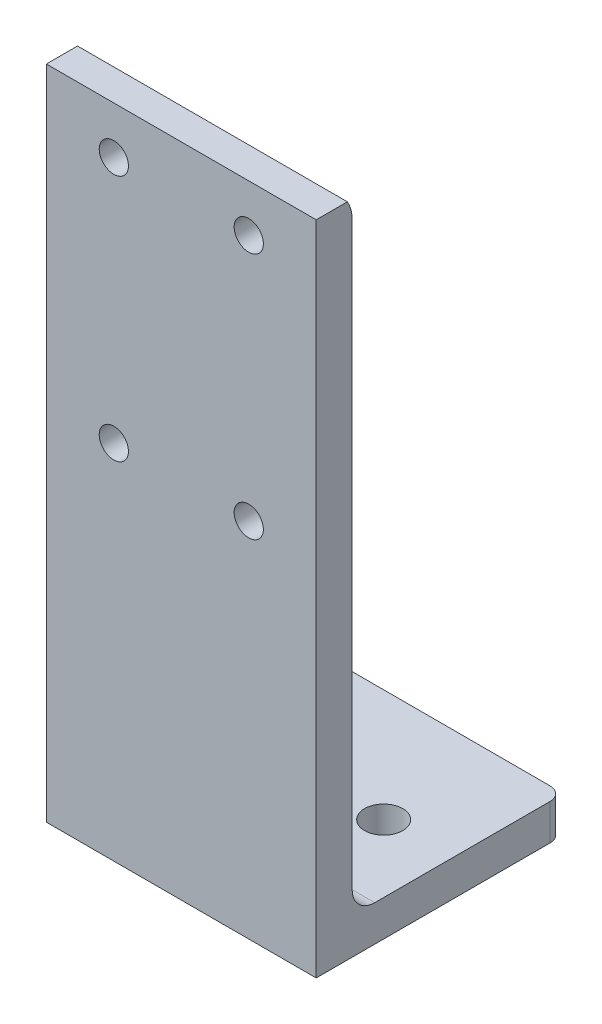
from build123d import *

# Parameters (mm, degrees)
MEMBER_1_DEPTH          = 60
SKETCH_3_W              = 60
SKETCH_3_H              = 15
CUT_EXTRUDE_1_DEPTH     = 177.068168617
SKETCH_4_W              = 60
SKETCH_4_H              = 4
CUT_EXTRUDE_2_DEPTH     = 171.660481659
HOLE_WIZARD_6_5_6_5_1_D = 6.5
FILLET_1_R              = 3
HOLE_WIZARD_8_5_8_5_1_D = 8.5


with BuildPart() as part:
    # Sketch1 → Member 1 (new body)
    with BuildSketch(Plane(origin=(0, 0, 0), x_dir=(0, 0, -1), z_dir=(1, 0, 0))):
        with BuildLine():
            Line((0, 0), (0, 150))
            ThreePointArc((0, 150), (5.656854249, 147.656854249), (8, 142))
            Line((8, 142), (8, 13))
            ThreePointArc((8, 13), (9.464466094, 9.464466094), (13, 8))
            Line((13, 8), (62, 8))
            ThreePointArc((62, 8), (67.656854249, 5.656854249), (70, 0))
            Line((70, 0), (0, 0))
        make_face()
    extrude(amount=MEMBER_1_DEPTH)

    # 草图3 → 切除-拉伸1 (cut, through all)
    with BuildSketch(Plane.XZ):
        with Locations((30, -62.5)):
            Rectangle(SKETCH_3_W, SKETCH_3_H)
    extrude(amount=-CUT_EXTRUDE_1_DEPTH, mode=Mode.SUBTRACT)

    # 草图4 → 切除-拉伸2 (cut, through all)
    with BuildSketch(Plane.XY):
        with Locations((30, 148)):
            Rectangle(SKETCH_4_W, SKETCH_4_H)
    extrude(amount=-CUT_EXTRUDE_2_DEPTH, mode=Mode.SUBTRACT)

    # Ø6.5 (6.5) 直径孔1 (through all)
    with Locations(Plane(origin=(0, 0, -8), x_dir=(-1, 0, 0), z_dir=(0, 0, -1))):
        with Locations((-45, 135.5), (-15, 135.5), (-45, 80.5), (-15, 80.5)):
            Hole(HOLE_WIZARD_6_5_6_5_1_D / 2)

    # 圆角1
    fillet_1_edges = [part.edges().sort_by_distance(p)[0] for p in [
        (0, 4, -55),
        (60, 4, -55),
    ]]
    fillet(fillet_1_edges, radius=FILLET_1_R)

    # Ø8.5 (8.5) 直径孔1 (through all)
    with Locations(Plane(origin=(0, 8, 0), x_dir=(1, 0, 0), z_dir=(0, 1, 0))):
        with Locations((15, 30), (45, 30)):
            Hole(HOLE_WIZARD_8_5_8_5_1_D / 2)


solid = part.part
